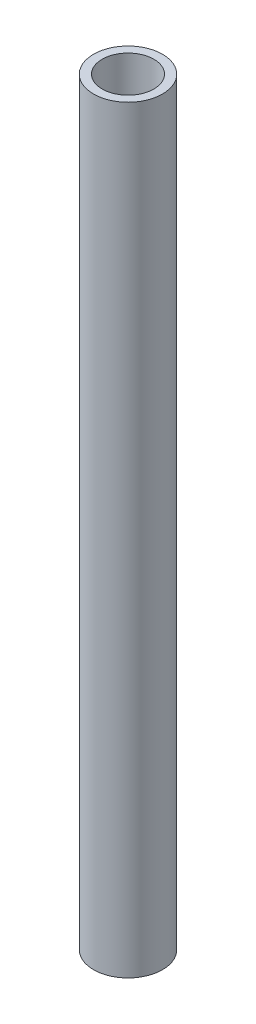
SolidWorks part; units mm, degrees
material "黄铜"
ref_plane "Front Plane" through (0, 0, 0) normal (0, 0, 1) x (1, 0, 0)
ref_plane "Top Plane" through (0, 0, 0) normal (0, 1, 0) x (1, 0, 0)
ref_plane "Right Plane" through (0, 0, 0) normal (1, 0, 0) x (0, 0, -1)
sketch "Sketch1" plane through (0, 0, 0) normal (0, 0, 1) x (1, 0, 0)
  line L0 (0, -14.4335) -> (0, 9.4598) construction
  line L1 (-0.75, 10.2) -> (-0.75, -11.8)
  line L2 (-1, 10.2) -> (-0.75, 10.2)
  line L3 (-1, -11.8) -> (-0.75, -11.8)
  line L6 (-1, 10.2) -> (-1, -11.8)
  dimension "D1" = 0.25
  dimension "D2" = 2
  dimension "D3" = 22
revolve "Revolve1" add sketch "Sketch1" angle 360 about L0
